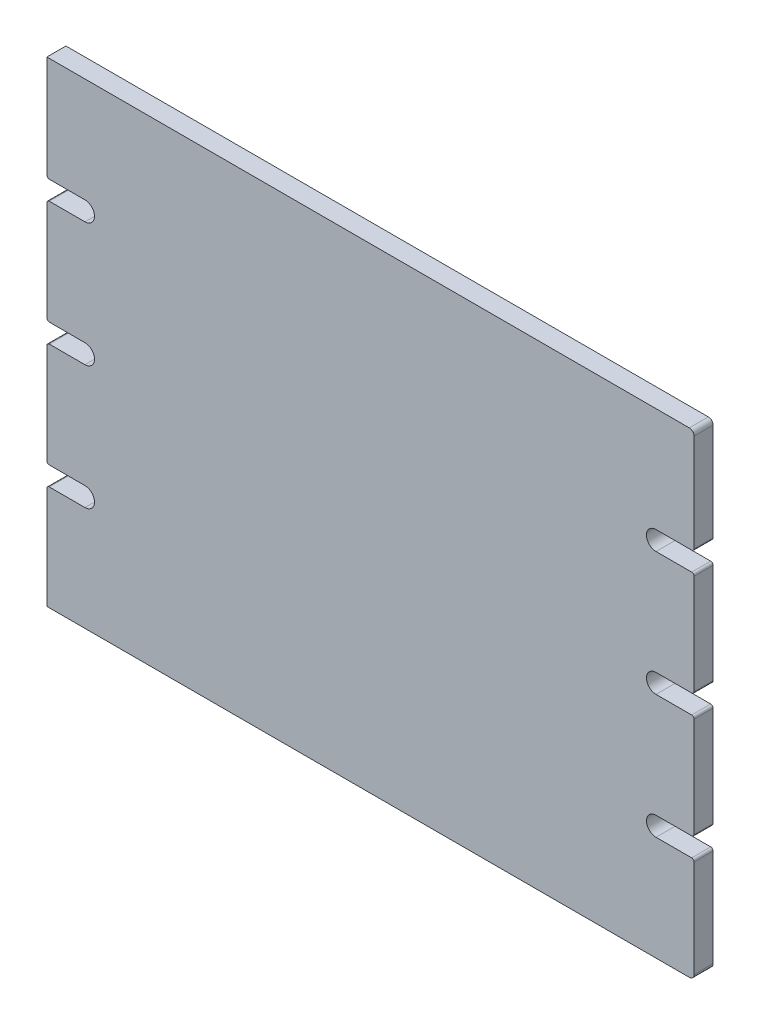
from build123d import *

# Parameters (mm, degrees)
BOSS_EXTRUDE1_DEPTH = 40
FILLET1_R           = 5
FILLET2_R           = 10


with BuildPart() as part:
    # Sketch1 → Boss-Extrude1 (new body)
    with BuildSketch(Plane.XY):
        with BuildLine():
            Line((0, 780), (80, 780))
            ThreePointArc((80, 780), (100, 760), (80, 740))
            Line((80, 740), (0, 740))
            Line((0, 740), (0, 520))
            Line((0, 520), (80, 520))
            ThreePointArc((80, 520), (100, 500), (80, 480))
            Line((80, 480), (0, 480))
            Line((0, 480), (0, 260))
            Line((0, 260), (80, 260))
            ThreePointArc((80, 260), (100, 240), (80, 220))
            Line((80, 220), (0, 220))
            Line((0, 220), (0, 0))
            Line((0, 0), (1360, 0))
            Line((1360, 0), (1360, 220))
            Line((1360, 220), (1280, 220))
            ThreePointArc((1280, 220), (1260, 240), (1280, 260))
            Line((1280, 260), (1360, 260))
            Line((1360, 260), (1360, 480))
            Line((1360, 480), (1280, 480))
            ThreePointArc((1280, 480), (1260, 500), (1280, 520))
            Line((1280, 520), (1360, 520))
            Line((1360, 520), (1360, 740))
            Line((1360, 740), (1280, 740))
            ThreePointArc((1280, 740), (1260, 760), (1280, 780))
            Line((1280, 780), (1360, 780))
            Line((1360, 780), (1360, 1000))
            Line((1360, 1000), (0, 1000))
            Line((0, 1000), (0, 780))
        make_face()
    extrude(amount=BOSS_EXTRUDE1_DEPTH)

    # Fillet1
    fillet1_edges = [part.edges().sort_by_distance(p)[0] for p in [
        (0, 220, 20),
        (0, 260, 20),
        (0, 480, 20),
        (0, 520, 20),
        (0, 740, 20),
        (0, 780, 20),
        (1360, 780, 20),
        (1360, 740, 20),
        (1360, 520, 20),
        (1360, 480, 20),
        (1360, 260, 20),
        (1360, 220, 20),
    ]]
    fillet(fillet1_edges, radius=FILLET1_R)

    # Fillet2
    fillet2_edges = [part.edges().sort_by_distance(p)[0] for p in [
        (1360, 1000, 20),
        (1360, 0, 20),
    ]]
    fillet(fillet2_edges, radius=FILLET2_R)


solid = part.part
